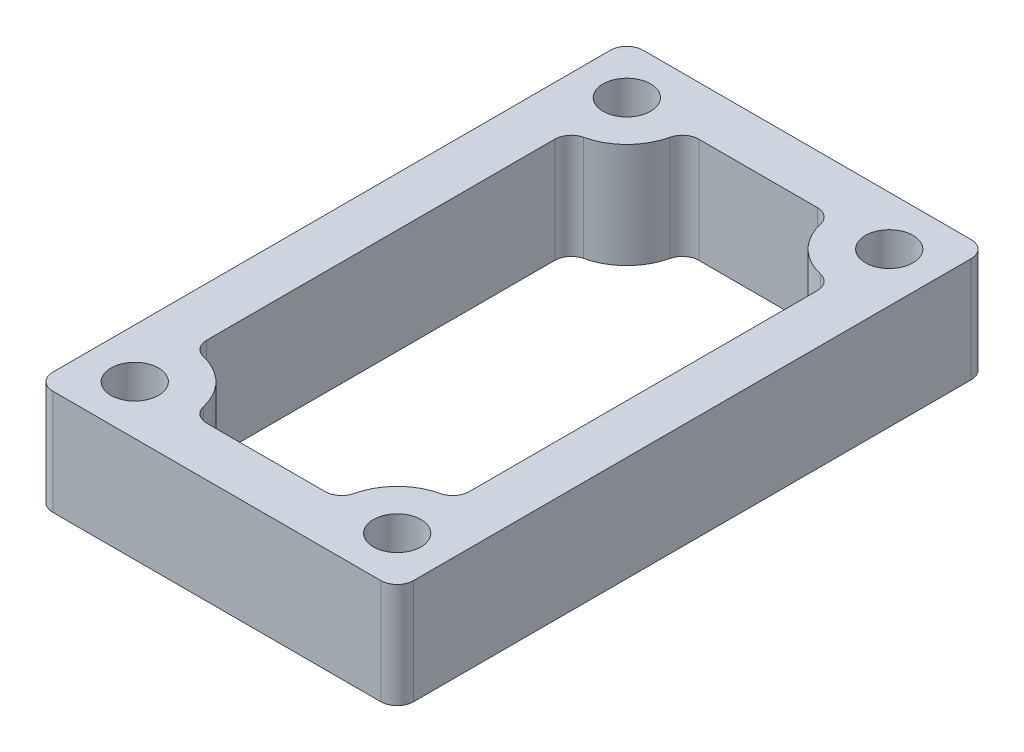
SolidWorks part; units mm, degrees
material "ABS"
ref_plane "前视基准面" through (0, 0, 0) normal (0, 0, 1) x (1, 0, 0)
ref_plane "上视基准面" through (0, 0, 0) normal (0, 1, 0) x (1, 0, 0)
ref_plane "右视基准面" through (0, 0, 0) normal (1, 0, 0) x (0, 0, -1)
sketch "草图1" plane through (0, 0, 0) normal (0, 1, 0) x (1, 0, 0)
  line L1 (8, -15) -> (-8, -15) construction
  line L2 (8, -15) -> (8, 15) construction
  line L3 (8, 15) -> (-8, 15) construction
  line L4 (-8, -15) -> (-8, 15) construction
  line L5 (8, -15) -> (-8, 15) construction
  line L6 (8, 15) -> (-8, -15) construction
  line L7 (11, -18) -> (-11, -18)
  line L8 (11, -18) -> (11, 18)
  line L9 (11, 18) -> (-11, 18)
  line L10 (-11, -18) -> (-11, 18)
  line L11 (11, -18) -> (-11, 18) construction
  line L12 (11, 18) -> (-11, -18) construction
  line L24 (-4.5, 15) -> (4.5, 15)
  line L25 (8, 11.5) -> (8, -11.5)
  line L26 (-8, 11.5) -> (-8, -11.5)
  line L27 (-4.5, -15) -> (4.5, -15)
  circle A0 centre (-8, 15) radius 1.45
  circle A1 centre (8, 15) radius 1.45
  circle A2 centre (-8, -15) radius 1.45
  circle A3 centre (8, -15) radius 1.45
  arc A4 (4.5, 15) -> (8, 11.5) centre (8, 15) ccw
  arc A5 (-4.5, 15) -> (-8, 11.5) centre (-8, 15) cw
  arc A6 (-8, -11.5) -> (-4.5, -15) centre (-8, -15) cw
  arc A7 (8, -11.5) -> (4.5, -15) centre (8, -15) ccw
  point P0 (0, 0)
  point P6 (0, 0)
  point P23 (0, 0)
  point P30 (0, 0)
  dimension "D1" = 2.9
  dimension "D7" = 3.5
  dimension "D2" = 16
  dimension "D3" = 30
  dimension "D4" = 3
  dimension "D5" = 3
  dimension "D6" = 3
  dimension "D8" = 3
  dimension "D9" = 3
  dimension "D10" = 3
extrude "凸台-拉伸1" add sketch "草图1" along normal blind 6.4 contours L10 L7 L8 L9 A3 A2 A1 A0
fillet "圆角1" radius 1 8 edges at (-4.5, 3.2, -15) (-4.5, 3.2, 15) (-8, 3.2, 11.5) (4.5, 3.2, 15) (8, 3.2, 11.5) (8, 3.2, -11.5) (4.5, 3.2, -15) (-8, 3.2, -11.5)
fillet "圆角2" radius 1 4 edges at (-11, 3.2, 18) (11, 3.2, 18) (11, 3.2, -18) (-11, 3.2, -18)
